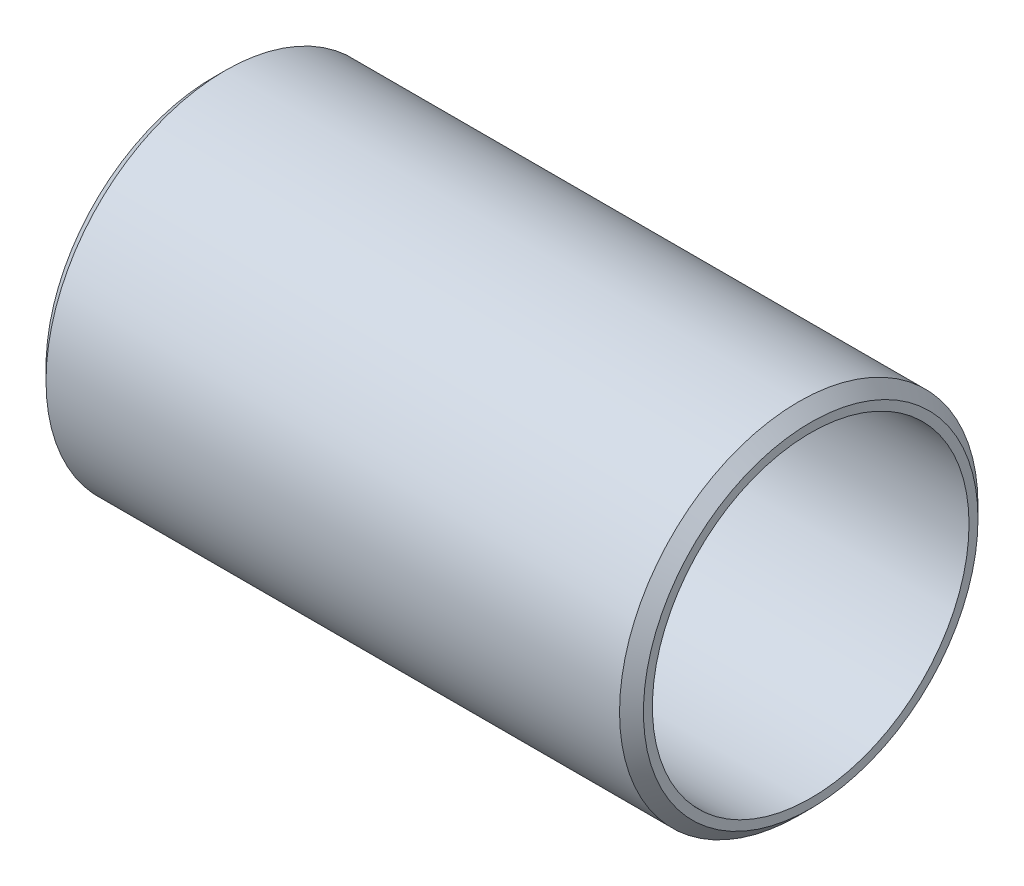
from build123d import *

# Parameters (mm, degrees)
SKETCH_1_R      = 30
SKETCH_1_R_2    = 26.5
EXTRUDE_1_DEPTH = 100
CHAMFER_1_SIZE  = 2


with BuildPart() as part:
    # 草图1 → 拉伸-薄壁1 (new body)
    with BuildSketch(Plane(origin=(0, 0, 0), x_dir=(0, 0, -1), z_dir=(1, 0, 0))):
        Circle(SKETCH_1_R)
        Circle(SKETCH_1_R_2, mode=Mode.SUBTRACT)
    extrude(amount=EXTRUDE_1_DEPTH)

    # 倒角1
    chamfer_1_edges = [part.edges().sort_by_distance(p)[0] for p in [
        (0, 0, 30),
        (100, 0, 30),
    ]]
    chamfer(chamfer_1_edges, length=CHAMFER_1_SIZE)


solid = part.part
